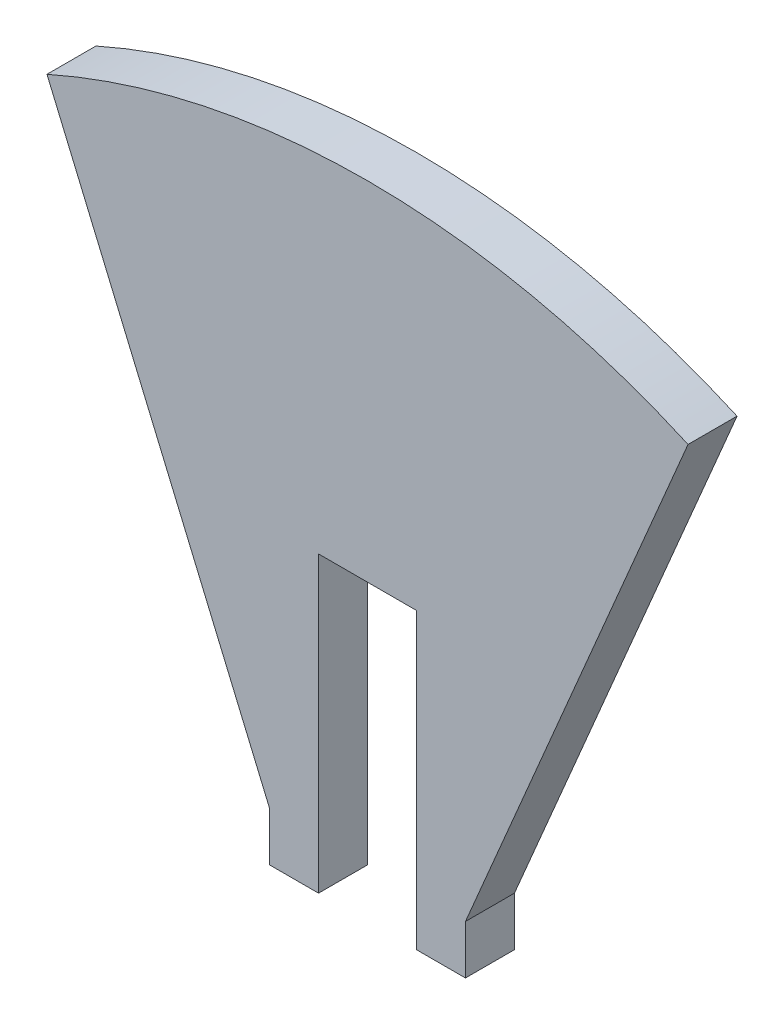
from build123d import *

# Parameters (mm, degrees)
BOSS_EXTRUDE1_DEPTH = 5
SKETCH2_W           = 20
SKETCH2_H           = 120
CUT_EXTRUDE1_DEPTH  = 10


with BuildPart() as part:
    # Sketch1 → Boss-Extrude1 (new, symmetric)
    with BuildSketch(Plane.XY):
        with BuildLine():
            Line((-65.458114903, 147.092607541), (-20, 40))
            Line((-20, 40), (-20, 30))
            Line((-20, 30), (20, 30))
            Line((20, 30), (20, 40))
            Line((20, 40), (65.458114903, 147.092607541))
            ThreePointArc((65.458114903, 147.092607541), (0, 161), (-65.458114903, 147.092607541))
        make_face()
    extrude(amount=BOSS_EXTRUDE1_DEPTH, both=True)

    # Sketch2 → Cut-Extrude1 (cut)
    with BuildSketch(Plane.XY.offset(5)):
        with Locations((0, 30)):
            Rectangle(SKETCH2_W, SKETCH2_H)
    extrude(amount=-CUT_EXTRUDE1_DEPTH, mode=Mode.SUBTRACT)


solid = part.part
